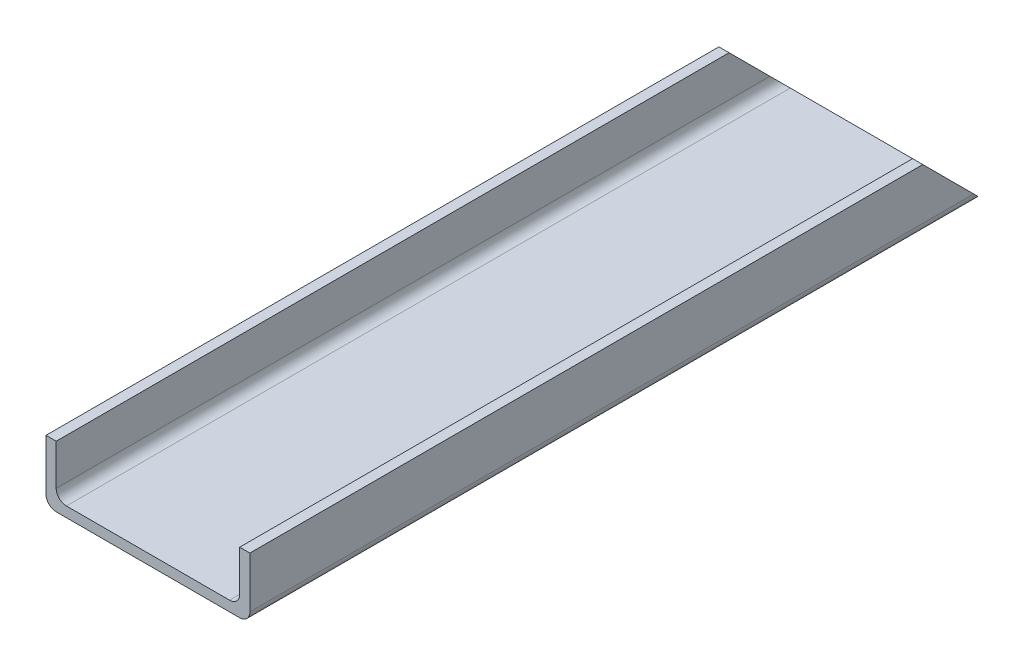
from build123d import *

# Parameters (mm, degrees)
EXTRUDE_1_DEPTH     = 360
CUT_EXTRUDE_1_DEPTH = 375.83329628


with BuildPart() as part:
    # 草图1 → 凸台-拉伸1 (new body)
    with BuildSketch(Plane.XY):
        with BuildLine():
            Line((5, 0), (95, 0))
            ThreePointArc((95, 0), (98.535533906, 1.464466094), (100, 5))
            Line((100, 5), (100, 30))
            Line((100, 30), (95, 30))
            Line((95, 30), (95, 10))
            ThreePointArc((95, 10), (93.535533906, 6.464466094), (90, 5))
            Line((90, 5), (10, 5))
            ThreePointArc((10, 5), (6.464466094, 6.464466094), (5, 10))
            Line((5, 10), (5, 30))
            Line((5, 30), (0, 30))
            Line((0, 30), (0, 5))
            ThreePointArc((0, 5), (1.464466094, 1.464466094), (5, 0))
        make_face()
    extrude(amount=EXTRUDE_1_DEPTH)

    # 草图2 → 切除-拉伸1 (cut, through all)
    with BuildSketch(Plane.ZY):
        Polygon((5, 5), (30, 30), (0, 30), (0, 5), align=None)
        Polygon((0, 0), (5, 5), (0, 5), align=None)
    extrude(amount=-CUT_EXTRUDE_1_DEPTH, mode=Mode.SUBTRACT)


solid = part.part
